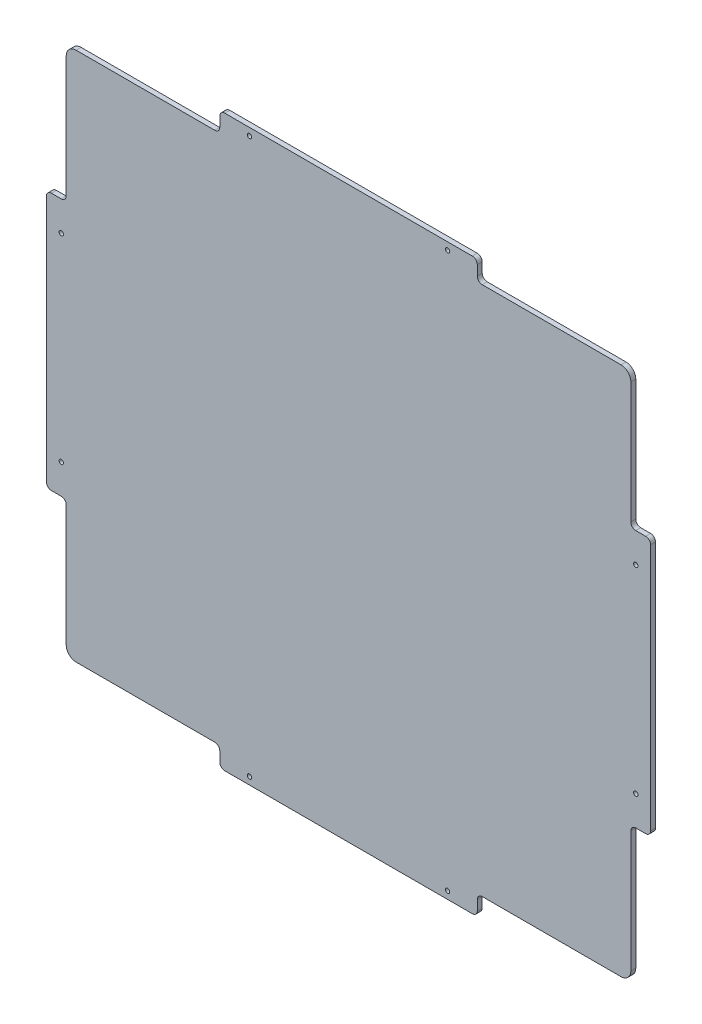
from build123d import *

# Parameters (mm, degrees)
SKETCH_1_W          = 570
SKETCH_1_H          = 535
EXTRUDE_1_DEPTH     = 5
FILLET_1_R          = 10
SKETCH_4_W          = 260
SKETCH_4_H          = 20
SKETCH_4_W_2        = 20
SKETCH_4_H_2        = 260
EXTRUDE_2_DEPTH     = 5
SKETCH_5_R          = 2.2
CUT_EXTRUDE_2_DEPTH = 420.17329352
FILLET_2_R          = 5


with BuildPart() as part:
    # 草图1 → 凸台-拉伸1 (new body)
    with BuildSketch(Plane.XY):
        Rectangle(SKETCH_1_W, SKETCH_1_H)
    extrude(amount=EXTRUDE_1_DEPTH)

    # 圆角1
    fillet_1_edges = [part.edges().sort_by_distance(p)[0] for p in [
        (285, -267.5, 2.5),
        (-285, -267.5, 2.5),
        (-285, 267.5, 2.5),
        (285, 267.5, 2.5),
    ]]
    fillet(fillet_1_edges, radius=FILLET_1_R)

    # 草图4 → 凸台-拉伸2 (add)
    with BuildSketch(Plane(origin=(0, 0, 0), x_dir=(-1, 0, 0), z_dir=(0, 0, -1))):
        with Locations((0, 277.5)):
            Rectangle(SKETCH_4_W, SKETCH_4_H)
        with Locations((295, 0)):
            Rectangle(SKETCH_4_W_2, SKETCH_4_H_2)
        with Locations((0, -277.5)):
            Rectangle(SKETCH_4_W, SKETCH_4_H)
        with Locations((-295, 0)):
            Rectangle(SKETCH_4_W_2, SKETCH_4_H_2)
    extrude(amount=-EXTRUDE_2_DEPTH)

    # 草图5 → 切除-拉伸2 (cut, through all)
    with BuildSketch(Plane(origin=(0, 0, 0), x_dir=(-1, 0, 0), z_dir=(0, 0, -1))):
        with Locations((-100, 280)):
            Circle(SKETCH_5_R)
        with Locations(Location((100, 280, 0), (0, 0, 180))):
            Circle(SKETCH_5_R)
        with Locations((290, 100)):
            Circle(SKETCH_5_R)
        with Locations(Location((290, -100, 0), (0, 0, 180))):
            Circle(SKETCH_5_R)
        with Locations((100, -280)):
            Circle(SKETCH_5_R)
        with Locations(Location((-100, -280, 0), (0, 0, 180))):
            Circle(SKETCH_5_R)
        with Locations((-290, -100)):
            Circle(SKETCH_5_R)
        with Locations(Location((-290, 100, 0), (0, 0, 180))):
            Circle(SKETCH_5_R)
    extrude(amount=-CUT_EXTRUDE_2_DEPTH, mode=Mode.SUBTRACT)

    # 圆角2
    fillet_2_edges = [part.edges().sort_by_distance(p)[0] for p in [
        (130, 287.5, 2.5),
        (130, 267.5, 2.5),
        (-130, 267.5, 2.5),
        (-130, 287.5, 2.5),
        (-305, -130, 2.5),
        (-305, 130, 2.5),
        (-285, 130, 2.5),
        (-285, -130, 2.5),
        (-130, -287.5, 2.5),
        (-130, -267.5, 2.5),
        (130, -267.5, 2.5),
        (130, -287.5, 2.5),
        (285, -130, 2.5),
        (285, 130, 2.5),
        (305, 130, 2.5),
        (305, -130, 2.5),
    ]]
    fillet(fillet_2_edges, radius=FILLET_2_R)


solid = part.part
